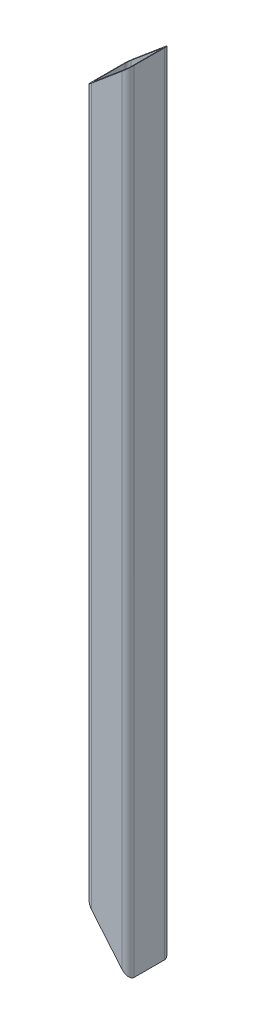
SolidWorks part; units mm, degrees
material "Q235B"
ref_plane "Front Plane" through (0, 0, 0) normal (0, 0, 1) x (1, 0, 0)
ref_plane "Top Plane" through (0, 0, 0) normal (0, 1, 0) x (1, 0, 0)
ref_plane "Right Plane" through (0, 0, 0) normal (1, 0, 0) x (0, 0, -1)
sketch "18 (ProfileFeature) (+7 more in 7 files) Sketch1" plane through (0, 0, 0) normal (0, 0, 1) x (1, 0, 0)
  line L0 (0, 0) -> (0, 1302)
  dimension "D1" = 1302
other "19 (WeldMemberFeat) (+4 more in 5 files) Cold-formed hollow square steel (GB/T 6728-2002) 70×70×5(1)"
ref_plane "Plane1" through (0, 0, 0) normal (0, 1, 0) x (-1, 0, 0)
sketch "Sketch1" plane through (0, 0, 0) normal (0, 1, 0) x (-1, 0, 0)
  line L0 (-25, -30) -> (25, -30)
  line L1 (-30, -25) -> (-30, 25)
  line L2 (25, 30) -> (-25, 30)
  line L3 (30, 25) -> (30, -25)
  line L4 (-25, -35) -> (25, -35)
  line L5 (-35, -25) -> (-35, 25)
  line L6 (25, 35) -> (-25, 35)
  line L7 (35, 25) -> (35, -25)
  arc A0 (35, 25) -> (25, 35) centre (25, 25) ccw
  arc A1 (25, -35) -> (35, -25) centre (25, -25) ccw
  arc A2 (-35, -25) -> (-25, -35) centre (-25, -25) ccw
  arc A3 (-25, 35) -> (-35, 25) centre (-25, 25) ccw
  arc A4 (-25, 30) -> (-30, 25) centre (-25, 25) ccw
  arc A5 (30, 25) -> (25, 30) centre (25, 25) ccw
  arc A6 (25, -30) -> (30, -25) centre (25, -25) ccw
  arc A7 (-30, -25) -> (-25, -30) centre (-25, -25) ccw
  point P0 (-35, 0)
  point P1 (35, 0)
  point P2 (0, 35)
  point P3 (0, -35)
  point P4 (0, 0)
  point P5 (-35, -35)
  point P6 (35, -35)
  point P7 (35, 35)
  point P8 (-35, 35)
  point P33 (0, 0)
  dimension "D1" = 10
  dimension "D2" = 70
  dimension "D3" = 5
sketch "Sketch2" plane through (0, 0, 35) normal (0, 0, 1) x (1, 0, 0)
  line L0 (35, 1302) -> (-35, 1243.247)
  line L1 (-35, 1302) -> (-35, 0) construction
  line L2 (-35, 1243.247) -> (-35, 1302)
  line L3 (-35, 1302) -> (35, 1302)
  line L4 (-35, 83.4) -> (35, 0)
  line L5 (35, 0) -> (-35, 0)
  line L6 (-35, 0) -> (-35, 83.4)
  dimension "D1" = 83.4
  dimension "D2" = 90
extrude "Cut-Extrude1" cut sketch "Sketch2" against normal through all both and the other way through all
